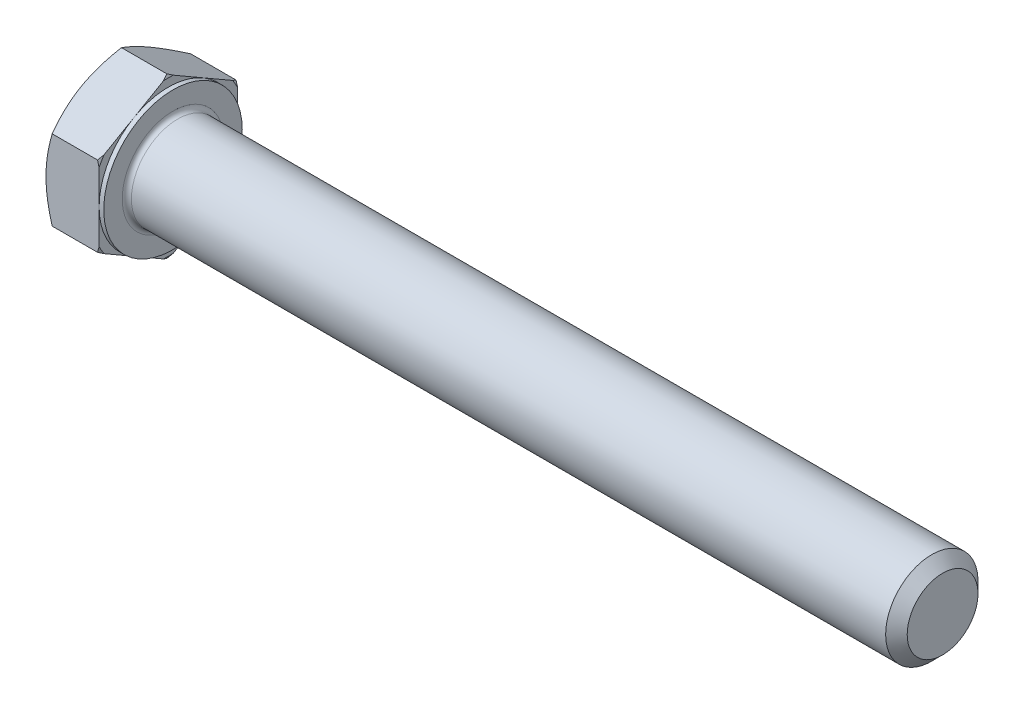
from build123d import *

# Parameters (mm, degrees)
BASE_EXTRUDE_DEPTH = 7.5
SKETCH4_W          = 0.6
SKETCH4_H          = 11.392304845
CHAMFER_2_SIZE     = 1.4
FILLET_2_R         = 0.6


with BuildPart() as part:
    # Sketch1 → Base-extrude (new body)
    with BuildSketch(Plane(origin=(0, 0, 0), x_dir=(0, 0, -1), z_dir=(1, 0, 0))):
        Polygon((9, 5.196152423), (9, -5.196152423), (0, -10.392304845), (-9, -5.196152423), (-9, 5.196152423), (0, 10.392304845), align=None)
    extrude(amount=BASE_EXTRUDE_DEPTH)

    # Sketch2 → Boss-Revolve1 (revolve)
    with BuildSketch(Plane.XY, mode=Mode.PRIVATE) as boss_revolve1_sk:
        Polygon((0, 0), (107.5, 0), (107.5, 4.4845), (107.5, 6), (7.791693541, 6), (0, 6), align=None)
    revolve(boss_revolve1_sk.sketch.rotate(Axis((0, 0, 0), (1, 0, 0)), 90), axis=Axis((0, 0, 0), (1, 0, 0)))

    # Sketch3 → Cut-Revolve1 (revolve, cut)
    with BuildSketch(Plane.XY):
        Polygon((0, 9), (3.690598923, 15.392304845), (3.690598923, 20.392304845), (-10, 20.392304845), (-10, 9), align=None)
    revolve(axis=Axis((0, 0, 0), (1, 0, 0)), mode=Mode.SUBTRACT)

    # Sketch5 → Cut-Revolve2 (revolve, cut)
    with BuildSketch(Plane.XY):
        Polygon((7.5, 9), (3.809401077, 15.392304845), (3.809401077, 20.392304845), (13.809401077, 20.392304845), (13.809401077, 9), align=None)
    revolve(axis=Axis((0, 0, 0), (1, 0, 0)), mode=Mode.SUBTRACT)

    # Sketch4 → Cut-Revolve3 (revolve, cut)
    with BuildSketch(Plane.XY, mode=Mode.PRIVATE) as cut_revolve3_sk:
        with Locations((7.2, 14.696152423)):
            Rectangle(SKETCH4_W, SKETCH4_H)
    revolve(cut_revolve3_sk.sketch.rotate(Axis((0, 0, 0), (1, 0, 0)), 270), axis=Axis((0, 0, 0), (1, 0, 0)), mode=Mode.SUBTRACT)

    # Chamfer 2
    chamfer_2_edges = [part.edges().sort_by_distance(p)[0] for p in [
        (107.5, 0, -6),
    ]]
    chamfer(chamfer_2_edges, length=CHAMFER_2_SIZE)

    # Fillet 2
    fillet_2_edges = [part.edges().sort_by_distance(p)[0] for p in [
        (7.5, 0, -6),
    ]]
    fillet(fillet_2_edges, radius=FILLET_2_R)


solid = part.part
